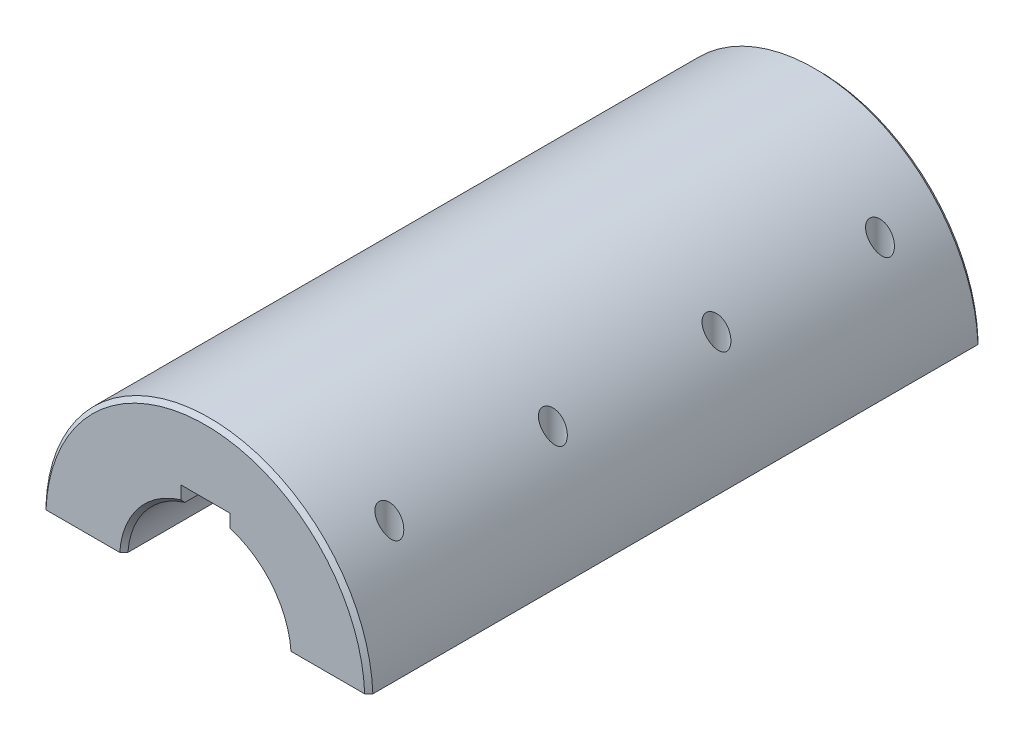
from build123d import *

# Parameters (mm, degrees)
SKETCH1_R            = 40
BOSS_EXTRUDE1_DEPTH  = 75
CHAMFER1_SIZE        = 1
SKETCH2_W            = 82
SKETCH2_H            = 3
CUT_EXTRUDE1_DEPTH   = 170
LPATTERN1_COUNT      = 4
LPATTERN1_PITCH      = 40
LPATTERN1_COUNT_DIR2 = 2
LPATTERN1_PITCH_DIR2 = 60


with BuildPart() as part:
    # Sketch1 → Boss-Extrude1 (new, symmetric)
    with BuildSketch(Plane.XY):
        Circle(SKETCH1_R)
        with BuildLine():
            Line((-6, 23.3), (6, 23.3))
            Line((6, 23.3), (6, 19.078784028))
            ThreePointArc((6, 19.078784028), (0, -20), (-6, 19.078784028))
            Line((-6, 19.078784028), (-6, 23.3))
        make_face(mode=Mode.SUBTRACT)
    extrude(amount=BOSS_EXTRUDE1_DEPTH, both=True)

    # Chamfer1
    chamfer1_edges = [part.edges().sort_by_distance(p)[0] for p in [
        (-40, 0, -75),
        (-40, 0, 75),
        (0, -20, -75),
        (0, -20, 75),
    ]]
    chamfer(chamfer1_edges, length=CHAMFER1_SIZE)

    # Sketch2 → Cut-Extrude1 (cut)
    with BuildSketch(Plane.XY.offset(75)):
        Rectangle(SKETCH2_W, SKETCH2_H)
    extrude(amount=-CUT_EXTRUDE1_DEPTH, mode=Mode.SUBTRACT)


with BuildPart() as cut_extrude1_kept_piece:
    # of the separate pieces the step leaves, the one the design keeps (cut_extrude1_pieces_kept)
    add(part.part.solids().sort_by_distance((39.971865105, 1.5, -74))[0])

    # Sketch5 → M6 Tapped Hole1 (revolve, cut)
    with BuildSketch(Plane(origin=(30, 1.5, 60), x_dir=(0, 0, -1), z_dir=(1, 0, 0))):
        Polygon((0, 0), (0, 40.502151548), (2.5, 39), (2.5, 0), align=None)
    m6_tapped_hole1 = revolve(axis=Axis((30, -4.85, 60), (0, 1, 0)), mode=Mode.SUBTRACT)

    # LPattern1: M6 Tapped Hole1 4 × 2
    with Locations(*[(-j * LPATTERN1_PITCH_DIR2, 0, -i * LPATTERN1_PITCH) for i in range(LPATTERN1_COUNT) for j in range(LPATTERN1_COUNT_DIR2) if (i, j) != (0, 0)]):
        add(m6_tapped_hole1, mode=Mode.SUBTRACT)


solid = cut_extrude1_kept_piece.part
